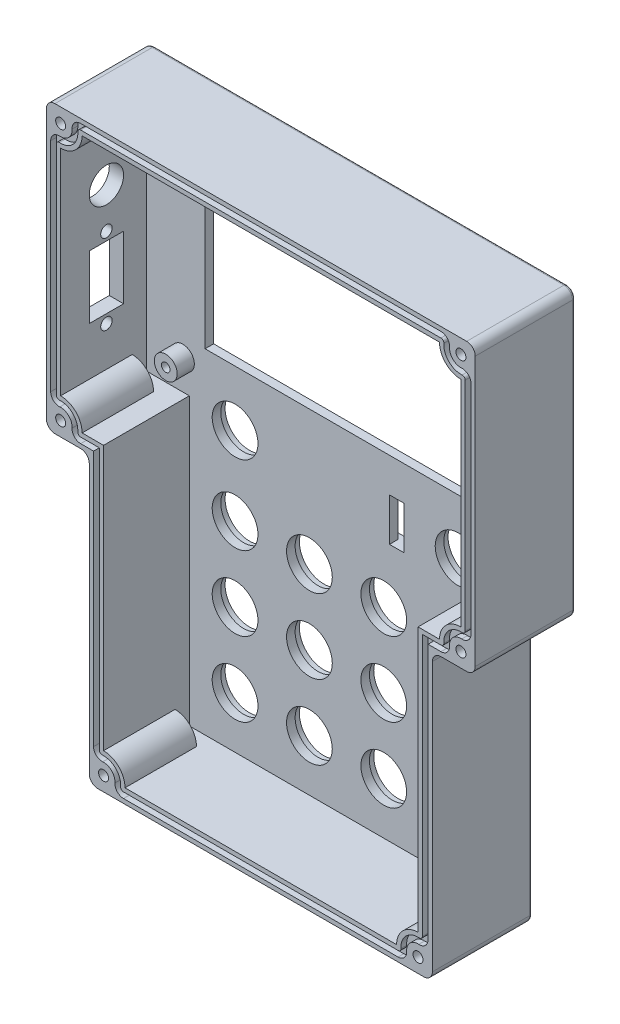
from build123d import *
from OCP.BRepFilletAPI import BRepFilletAPI_MakeChamfer

# Parameters (mm, degrees)
SKETCH1_R           = 8
SKETCH1_W           = 99
SKETCH1_H           = 58
BOSS_EXTRUDE1_DEPTH = 35
CUT_EXTRUDE1_DEPTH  = 30
FILLET1_R           = 3
FILLET2_R           = 1
SKETCH3_R           = 8.5
CUT_EXTRUDE2_DEPTH  = 2
CHAMFER1_SIZE       = 2
CHAMFER1_SIZE2      = 2.965121937
SKETCH5_R           = 4
SKETCH5_R_2         = 1.5
BOSS_EXTRUDE2_DEPTH = 6
BOSS_EXTRUDE3_DEPTH = 25
SKETCH7_R           = 1.75
CUT_EXTRUDE4_DEPTH  = 20
CUT_EXTRUDE5_DEPTH  = 2
SKETCH10_W          = 40
SKETCH10_H          = 15
CUT_EXTRUDE6_DEPTH  = 2
CUT_EXTRUDE7_REACH  = 218.134
SKETCH11_W          = 5
SKETCH11_H          = 15
CUT_EXTRUDE8_REACH  = 254.438
SKETCH12_R          = 6
SKETCH12_R_2        = 2
SKETCH12_W          = 12
SKETCH12_H          = 22


with BuildPart() as part:
    # Sketch1 → Boss-Extrude1 (new body)
    with BuildSketch(Plane.XY):
        Polygon((75, 200), (-75, 200), (-75, 100), (-60, 100), (-60, 0), (60, 0), (60, 100), (75, 100), align=None)
        with Locations((-13, 23)):
            Circle(SKETCH1_R, mode=Mode.SUBTRACT)
        with Locations((-39, 23)):
            Circle(SKETCH1_R, mode=Mode.SUBTRACT)
        with Locations((-39, 49)):
            Circle(SKETCH1_R, mode=Mode.SUBTRACT)
        with Locations((-13, 49)):
            Circle(SKETCH1_R, mode=Mode.SUBTRACT)
        with Locations((-39, 75)):
            Circle(SKETCH1_R, mode=Mode.SUBTRACT)
        with Locations((-13, 75)):
            Circle(SKETCH1_R, mode=Mode.SUBTRACT)
        with Locations((-39, 102.5)):
            Circle(SKETCH1_R, mode=Mode.SUBTRACT)
        with Locations(Location((13, 75, 0), (0, 0, 180))):
            Circle(SKETCH1_R, mode=Mode.SUBTRACT)
        with Locations(Location((39, 75, 0), (0, 0, 180))):
            Circle(SKETCH1_R, mode=Mode.SUBTRACT)
        with Locations(Location((13, 49, 0), (0, 0, 180))):
            Circle(SKETCH1_R, mode=Mode.SUBTRACT)
        with Locations(Location((39, 49, 0), (0, 0, 180))):
            Circle(SKETCH1_R, mode=Mode.SUBTRACT)
        with Locations(Location((39, 23, 0), (0, 0, 180))):
            Circle(SKETCH1_R, mode=Mode.SUBTRACT)
        with Locations(Location((13, 23, 0), (0, 0, 180))):
            Circle(SKETCH1_R, mode=Mode.SUBTRACT)
        with Locations(Location((39, 102.5, 0), (0, 0, 180))):
            Circle(SKETCH1_R, mode=Mode.SUBTRACT)
        with Locations((0, 151)):
            Rectangle(SKETCH1_W, SKETCH1_H, mode=Mode.SUBTRACT)
    extrude(amount=BOSS_EXTRUDE1_DEPTH)

    # Sketch2 → Cut-Extrude1 (cut)
    with BuildSketch(Plane.XY.offset(35)):
        Polygon((70, 105), (70, 195), (-70, 195), (-70, 105), (-55, 105), (-55, 5), (55, 5), (55, 105), align=None)
    extrude(amount=-CUT_EXTRUDE1_DEPTH, mode=Mode.SUBTRACT)

    # Fillet1
    fillet1_edges = [part.edges().sort_by_distance(p)[0] for p in [
        (-75, 100, 17.5),
        (-75, 200, 17.5),
        (75, 200, 17.5),
        (75, 100, 17.5),
        (60, 100, 17.5),
        (60, 0, 17.5),
        (-60, 0, 17.5),
        (-60, 100, 17.5),
    ]]
    fillet(fillet1_edges, radius=FILLET1_R)

    # Fillet2
    fillet2_edges = [part.edges().sort_by_distance(p)[0] for p in [
        (67.5, 100, 0),
        (60, 50, 0),
        (-60, 50, 0),
        (-67.5, 100, 0),
        (0, 0, 0),
        (-75, 150, 0),
        (0, 200, 0),
        (75, 150, 0),
        (-74.121320344, 199.121320344, 0),
        (-74.121320344, 100.878679656, 0),
        (74.121320344, 199.121320344, 0),
        (74.121320344, 100.878679656, 0),
        (59.121320344, 0.878679656, 0),
        (-59.121320344, 0.878679656, 0),
        (60.878679656, 99.121320344, 0),
        (-60.878679656, 99.121320344, 0),
    ]]
    fillet(fillet2_edges, radius=FILLET2_R)

    # Sketch3 → Cut-Extrude2 (cut)
    with BuildSketch(Plane(origin=(0, 0, 0), x_dir=(-1, 0, 0), z_dir=(0, 0, -1))):
        with Locations((-39, 23)):
            Circle(SKETCH3_R)
        with Locations((-13, 23)):
            Circle(SKETCH3_R)
        with Locations((-13, 49)):
            Circle(SKETCH3_R)
        with Locations((-39, 49)):
            Circle(SKETCH3_R)
        with Locations((-39, 75)):
            Circle(SKETCH3_R)
        with Locations((-13, 75)):
            Circle(SKETCH3_R)
        with Locations((-39, 102.5)):
            Circle(SKETCH3_R)
        with Locations(Location((39, 102.5, 0), (0, 0, 180))):
            Circle(SKETCH3_R)
        with Locations(Location((13, 75, 0), (0, 0, 180))):
            Circle(SKETCH3_R)
        with Locations(Location((39, 75, 0), (0, 0, 180))):
            Circle(SKETCH3_R)
        with Locations(Location((39, 49, 0), (0, 0, 180))):
            Circle(SKETCH3_R)
        with Locations(Location((13, 49, 0), (0, 0, 180))):
            Circle(SKETCH3_R)
        with Locations(Location((13, 23, 0), (0, 0, 180))):
            Circle(SKETCH3_R)
        with Locations(Location((39, 23, 0), (0, 0, 180))):
            Circle(SKETCH3_R)
    extrude(amount=-CUT_EXTRUDE2_DEPTH, mode=Mode.SUBTRACT)

    # Chamfer1: one chamfer whose edges measure the first distance from different faces: ONE call of the kernel's chamfer builder (chamfer() names one face for all edges)
    chamfer1_edges_1 = [part.edges().sort_by_distance(p)[0] for p in [
        (49.5, 151, 0),
    ]]
    chamfer1_side_1 = [part.faces().sort_by_distance(p)[0] for p in [
        (49.5, 151, 2.5),
    ]]
    chamfer1_edges_2 = [part.edges().sort_by_distance(p)[0] for p in [
        (0, 180, 0),
    ]]
    chamfer1_side_2 = [part.faces().sort_by_distance(p)[0] for p in [
        (0, 180, 2.5),
    ]]
    chamfer1_edges_3 = [part.edges().sort_by_distance(p)[0] for p in [
        (-49.5, 151, 0),
    ]]
    chamfer1_side_3 = [part.faces().sort_by_distance(p)[0] for p in [
        (-49.5, 151, 2.5),
    ]]
    chamfer1_edges_4 = [part.edges().sort_by_distance(p)[0] for p in [
        (0, 122, 0),
    ]]
    chamfer1_side_4 = [part.faces().sort_by_distance(p)[0] for p in [
        (0, 122, 2.5),
    ]]
    chamfer1 = BRepFilletAPI_MakeChamfer(part.part.solid().wrapped)
    for e in chamfer1_edges_1:
        chamfer1.Add(CHAMFER1_SIZE, CHAMFER1_SIZE2, e.wrapped, chamfer1_side_1[0].wrapped)  # the first distance lies on this face
    for e in chamfer1_edges_2:
        chamfer1.Add(CHAMFER1_SIZE, CHAMFER1_SIZE2, e.wrapped, chamfer1_side_2[0].wrapped)  # the first distance lies on this face
    for e in chamfer1_edges_3:
        chamfer1.Add(CHAMFER1_SIZE, CHAMFER1_SIZE2, e.wrapped, chamfer1_side_3[0].wrapped)  # the first distance lies on this face
    for e in chamfer1_edges_4:
        chamfer1.Add(CHAMFER1_SIZE, CHAMFER1_SIZE2, e.wrapped, chamfer1_side_4[0].wrapped)  # the first distance lies on this face
    add(Compound.cast(chamfer1.Shape()), mode=Mode.REPLACE)

    # Sketch5 → Boss-Extrude2 (add)
    # profile 1 of 4: a face of its own
    with BuildSketch(Plane.XY.offset(5)):
        with Locations((-57.25, 181.5)):
            Circle(SKETCH5_R)
        with Locations((-57.25, 181.5)):
            Circle(SKETCH5_R_2, mode=Mode.SUBTRACT)
    # profile 2 of 4: a face of its own
    with BuildSketch(Plane.XY.offset(5)):
        with Locations((57.25, 181.5)):
            Circle(SKETCH5_R)
        with Locations((57.25, 181.5)):
            Circle(SKETCH5_R_2, mode=Mode.SUBTRACT)
    # profile 3 of 4: a face of its own
    with BuildSketch(Plane.XY.offset(5)):
        with Locations((-57.25, 115.5)):
            Circle(SKETCH5_R)
        with Locations((-57.25, 115.5)):
            Circle(SKETCH5_R_2, mode=Mode.SUBTRACT)
    # profile 4 of 4: a face of its own
    with BuildSketch(Plane.XY.offset(5)):
        with Locations((57.25, 115.5)):
            Circle(SKETCH5_R)
        with Locations((57.25, 115.5)):
            Circle(SKETCH5_R_2, mode=Mode.SUBTRACT)
    extrude(amount=BOSS_EXTRUDE2_DEPTH)

    # Sketch6 → Boss-Extrude3 (add)
    with BuildSketch(Plane.XY.offset(35)):
        with BuildLine():
            Line((-71.747064875, 196.748861378), (-62.706750801, 196.748861378))
            ThreePointArc((-62.706750801, 196.748861378), (-64.696046035, 189.697352328), (-71.747064875, 187.706320248))
            Line((-71.747064875, 187.706320248), (-71.747064875, 196.748861378))
        make_face()
        with BuildLine():
            Line((71.50031539, 195.771596957), (62.539796374, 195.771596957))
            ThreePointArc((62.539796374, 195.771596957), (64.963763881, 189.442453262), (71.50031539, 187.651595157))
            Line((71.50031539, 187.651595157), (71.50031539, 195.771596957))
        make_face()
        with BuildLine():
            Line((71.50031539, 103.139966112), (62.734308434, 103.139966112))
            ThreePointArc((62.734308434, 103.139966112), (64.567806467, 110.171196518), (71.50031539, 112.348404843))
            Line((71.50031539, 112.348404843), (71.50031539, 103.139966112))
        make_face()
        with BuildLine():
            Line((-56.424780788, 4.339960717), (-47.529099911, 4.339960717))
            ThreePointArc((-47.529099911, 4.339960717), (-49.976766301, 10.56930186), (-56.424780788, 12.363423097))
            Line((-56.424780788, 12.363423097), (-56.424780788, 4.339960717))
        make_face()
        with BuildLine():
            Line((56.315887188, 4.339960717), (47.529099911, 4.339960717))
            ThreePointArc((47.529099911, 4.339960717), (49.935780208, 10.532059101), (56.315887188, 12.3836604))
            Line((56.315887188, 12.3836604), (56.315887188, 4.339960717))
        make_face()
        with BuildLine():
            Line((-71.747064875, 102.631768342), (-62.883717346, 102.631768342))
            ThreePointArc((-62.883717346, 102.631768342), (-64.473223551, 110.069984427), (-71.747064875, 112.293679752))
            Line((-71.747064875, 112.293679752), (-71.747064875, 102.631768342))
        make_face()
    extrude(amount=-BOSS_EXTRUDE3_DEPTH)

    # Sketch7 → Cut-Extrude4 (cut)
    with BuildSketch(Plane.XY.offset(35)):
        with Locations((-70, 195)):
            Circle(SKETCH7_R)
        with Locations((-70, 105)):
            Circle(SKETCH7_R)
        with Locations((-55, 5)):
            Circle(SKETCH7_R)
        with Locations(Location((55, 5, 0), (0, 0, 180))):
            Circle(SKETCH7_R)
        with Locations(Location((70, 105, 0), (0, 0, 180))):
            Circle(SKETCH7_R)
        with Locations(Location((70, 195, 0), (0, 0, 180))):
            Circle(SKETCH7_R)
    extrude(amount=-CUT_EXTRUDE4_DEPTH, mode=Mode.SUBTRACT)

    # Sketch9 → Cut-Extrude5 (cut)
    with BuildSketch(Plane.XY.offset(35)):
        with BuildLine():
            Line((63.017879978, 198.5), (-63.017879978, 198.5))
            ThreePointArc((-63.017879978, 198.5), (-65.213655142, 197.544155432), (-66.01021713, 195.285714286))
            ThreePointArc((-66.01021713, 195.285714286), (-67.171572875, 192.171572875), (-70.285714286, 191.01021713))
            ThreePointArc((-70.285714286, 191.01021713), (-72.544155432, 190.213655142), (-73.5, 188.017879978))
            Line((-73.5, 188.017879978), (-73.5, 111.982120022))
            ThreePointArc((-73.5, 111.982120022), (-72.544155432, 109.786344858), (-70.285714286, 108.98978287))
            ThreePointArc((-70.285714286, 108.98978287), (-67.171572875, 107.828427125), (-66.01021713, 104.714285714))
            ThreePointArc((-66.01021713, 104.714285714), (-65.213655142, 102.455844568), (-63.017879978, 101.5))
            Line((-63.017879978, 101.5), (-58.5, 101.5))
            Line((-58.5, 101.5), (-58.5, 11.982120022))
            ThreePointArc((-58.5, 11.982120022), (-57.544155432, 9.786344858), (-55.285714286, 8.98978287))
            ThreePointArc((-55.285714286, 8.98978287), (-52.171572875, 7.828427125), (-51.01021713, 4.714285714))
            ThreePointArc((-51.01021713, 4.714285714), (-50.213655142, 2.455844568), (-48.017879978, 1.5))
            Line((-48.017879978, 1.5), (48.017879978, 1.5))
            ThreePointArc((48.017879978, 1.5), (50.213655142, 2.455844568), (51.01021713, 4.714285714))
            ThreePointArc((51.01021713, 4.714285714), (52.171572875, 7.828427125), (55.285714286, 8.98978287))
            ThreePointArc((55.285714286, 8.98978287), (57.544155432, 9.786344858), (58.5, 11.982120022))
            Line((58.5, 11.982120022), (58.5, 101.5))
            Line((58.5, 101.5), (63.017879978, 101.5))
            ThreePointArc((63.017879978, 101.5), (65.213655142, 102.455844568), (66.01021713, 104.714285714))
            ThreePointArc((66.01021713, 104.714285714), (67.171572875, 107.828427125), (70.285714286, 108.98978287))
            ThreePointArc((70.285714286, 108.98978287), (72.544155432, 109.786344858), (73.5, 111.982120022))
            Line((73.5, 111.982120022), (73.5, 188.017879978))
            ThreePointArc((73.5, 188.017879978), (72.544155432, 190.213655142), (70.285714286, 191.01021713))
            ThreePointArc((70.285714286, 191.01021713), (67.171572875, 192.171572875), (66.01021713, 195.285714286))
            ThreePointArc((66.01021713, 195.285714286), (65.213655142, 197.544155432), (63.017879978, 198.5))
        make_face()
        with BuildLine():
            Line((71.5, 111.982120022), (71.5, 188.017879978))
            ThreePointArc((71.5, 188.017879978), (71.181385144, 188.749805033), (70.428571429, 189.015325696))
            ThreePointArc((70.428571429, 189.015325696), (65.757359313, 190.757359313), (64.015325696, 195.428571429))
            ThreePointArc((64.015325696, 195.428571429), (63.749805033, 196.181385144), (63.017879978, 196.5))
            Line((63.017879978, 196.5), (-63.017879978, 196.5))
            ThreePointArc((-63.017879978, 196.5), (-63.749805033, 196.181385144), (-64.015325696, 195.428571429))
            ThreePointArc((-64.015325696, 195.428571429), (-65.757359313, 190.757359313), (-70.428571429, 189.015325696))
            ThreePointArc((-70.428571429, 189.015325696), (-71.181385144, 188.749805033), (-71.5, 188.017879978))
            Line((-71.5, 188.017879978), (-71.5, 111.982120022))
            ThreePointArc((-71.5, 111.982120022), (-71.181385144, 111.250194967), (-70.428571429, 110.984674304))
            ThreePointArc((-70.428571429, 110.984674304), (-65.757359313, 109.242640687), (-64.015325696, 104.571428571))
            ThreePointArc((-64.015325696, 104.571428571), (-63.749805033, 103.818614856), (-63.017879978, 103.5))
            Line((-63.017879978, 103.5), (-56.5, 103.5))
            Line((-56.5, 103.5), (-56.5, 11.982120022))
            ThreePointArc((-56.5, 11.982120022), (-56.181385144, 11.250194967), (-55.428571429, 10.984674304))
            ThreePointArc((-55.428571429, 10.984674304), (-50.757359313, 9.242640687), (-49.015325696, 4.571428571))
            ThreePointArc((-49.015325696, 4.571428571), (-48.749805033, 3.818614856), (-48.017879978, 3.5))
            Line((-48.017879978, 3.5), (48.017879978, 3.5))
            ThreePointArc((48.017879978, 3.5), (48.749805033, 3.818614856), (49.015325696, 4.571428571))
            ThreePointArc((49.015325696, 4.571428571), (50.757359313, 9.242640687), (55.428571429, 10.984674304))
            ThreePointArc((55.428571429, 10.984674304), (56.181385144, 11.250194967), (56.5, 11.982120022))
            Line((56.5, 11.982120022), (56.5, 103.5))
            Line((56.5, 103.5), (63.017879978, 103.5))
            ThreePointArc((63.017879978, 103.5), (63.749805033, 103.818614856), (64.015325696, 104.571428571))
            ThreePointArc((64.015325696, 104.571428571), (65.757359313, 109.242640687), (70.428571429, 110.984674304))
            ThreePointArc((70.428571429, 110.984674304), (71.181385144, 111.250194967), (71.5, 111.982120022))
        make_face(mode=Mode.SUBTRACT)
    extrude(amount=-CUT_EXTRUDE5_DEPTH, mode=Mode.SUBTRACT)

    # Sketch10 → Cut-Extrude6 (cut)
    with BuildSketch(Plane(origin=(0, 0, 0), x_dir=(-1, 0, 0), z_dir=(0, 0, -1))):
        with Locations((0, 102.5)):
            Rectangle(SKETCH10_W, SKETCH10_H)
    extrude(amount=-CUT_EXTRUDE6_DEPTH, mode=Mode.SUBTRACT)

    # Sketch11 → Cut-Extrude7 (cut, up to next)
    with BuildSketch(Plane(origin=(0, 0, 2), x_dir=(-1, 0, 0), z_dir=(0, 0, -1)), mode=Mode.PRIVATE) as cut_extrude7_sk1:
        with Locations((-17.5, 102.5)):
            Rectangle(SKETCH11_W, SKETCH11_H)
    cut_extrude7_tool1 = extrude(cut_extrude7_sk1.sketch, amount=-CUT_EXTRUDE7_REACH, mode=Mode.PRIVATE) & part.part
    add(cut_extrude7_tool1.solids().sort_by_distance((17.5, 102.5, 2))[0], mode=Mode.SUBTRACT)

    # Sketch12 → Cut-Extrude8 (cut, up to next)
    with BuildSketch(Plane.ZY.offset(75), mode=Mode.PRIVATE) as cut_extrude8_sk1:
        with Locations(Location((19, 168.38, 0), (0, 0, 270))):
            Circle(SKETCH12_R)
    cut_extrude8_tool1 = extrude(cut_extrude8_sk1.sketch, amount=-CUT_EXTRUDE8_REACH, mode=Mode.PRIVATE) & part.part
    # Sketch12 → Cut-Extrude8 (cut, up to next)
    with BuildSketch(Plane.ZY.offset(75), mode=Mode.PRIVATE) as cut_extrude8_sk2:
        with Locations(Location((19, 154.38, 0), (0, 0, 270))):
            Circle(SKETCH12_R_2)
    cut_extrude8_tool2 = extrude(cut_extrude8_sk2.sketch, amount=-CUT_EXTRUDE8_REACH, mode=Mode.PRIVATE) & part.part
    # Sketch12 → Cut-Extrude8 (cut, up to next)
    with BuildSketch(Plane.ZY.offset(75), mode=Mode.PRIVATE) as cut_extrude8_sk3:
        with Locations(Location((19, 126.38, 0), (0, 0, 270))):
            Circle(SKETCH12_R_2)
    cut_extrude8_tool3 = extrude(cut_extrude8_sk3.sketch, amount=-CUT_EXTRUDE8_REACH, mode=Mode.PRIVATE) & part.part
    # Sketch12 → Cut-Extrude8 (cut, up to next)
    with BuildSketch(Plane.ZY.offset(75), mode=Mode.PRIVATE) as cut_extrude8_sk4:
        with Locations((19, 140.38)):
            Rectangle(SKETCH12_W, SKETCH12_H)
    cut_extrude8_tool4 = extrude(cut_extrude8_sk4.sketch, amount=-CUT_EXTRUDE8_REACH, mode=Mode.PRIVATE) & part.part
    add(cut_extrude8_tool1.solids().sort_by_distance((-75, 168.38, 19))[0], mode=Mode.SUBTRACT)
    add(cut_extrude8_tool2.solids().sort_by_distance((-75, 154.38, 19))[0], mode=Mode.SUBTRACT)
    add(cut_extrude8_tool3.solids().sort_by_distance((-75, 126.38, 19))[0], mode=Mode.SUBTRACT)
    add(cut_extrude8_tool4.solids().sort_by_distance((-75, 140.38, 19))[0], mode=Mode.SUBTRACT)


solid = part.part
